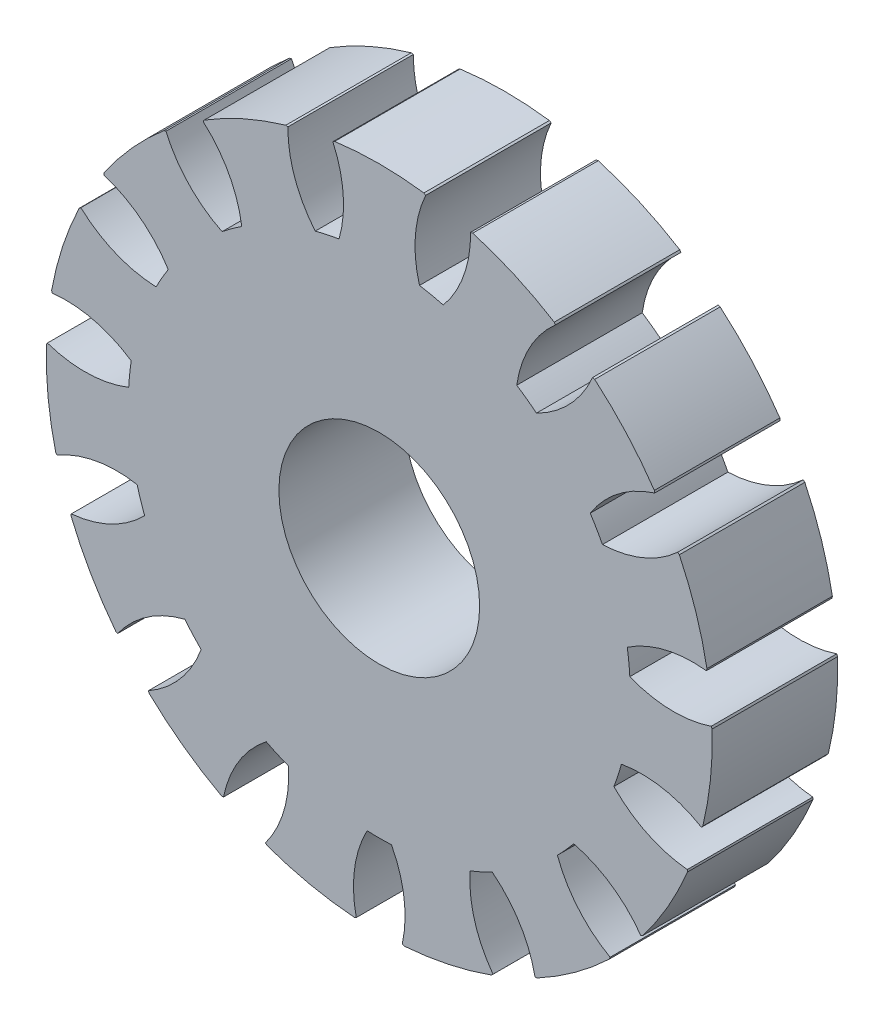
from build123d import *

# Parameters (mm, degrees)
SKETCH1_R           = 10
BOSS_EXTRUDE1_DEPTH = 5
SKETCH4_R           = 2.25
CUT_EXTRUDE2_DEPTH  = 67.5
BOSS_EXTRUDE3_DEPTH = 5
CIRPATTERN2_COUNT   = 15
SKETCH6_OUTSIDE_W   = 36.97
SKETCH6_OUTSIDE_H   = 36.858
SKETCH6_OUTSIDE_R   = 13.270335227
CUT_EXTRUDE3_DEPTH  = 20.926845935
SKETCH7_R           = 4
CUT_EXTRUDE4_DEPTH  = 20.421729945


with BuildPart() as part:
    # Sketch1 → Boss-Extrude1 (new body)
    with BuildSketch(Plane.XY):
        Circle(SKETCH1_R)
    extrude(amount=BOSS_EXTRUDE1_DEPTH)

    # Sketch4 → Cut-Extrude2 (cut, symmetric)
    with BuildSketch(Plane.XY):
        Circle(SKETCH4_R)
    extrude(amount=CUT_EXTRUDE2_DEPTH, both=True, mode=Mode.SUBTRACT)

    # Sketch5 → Boss-Extrude3 (add)
    with BuildSketch(Plane.XY):
        with BuildLine():
            ThreePointArc((1.602050877, 9.870837502), (0, 10), (-1.602050877, 9.870837502))
            ThreePointArc((-1.602050877, 9.870837502), (-1.43729136, 11.509422675), (-1.849699914, 13.103795985))
            ThreePointArc((-1.849699914, 13.103795985), (0, 13.667962875), (1.849699914, 13.103795985))
            ThreePointArc((1.849699914, 13.103795985), (1.43729136, 11.509422675), (1.602050877, 9.870837502))
        make_face()
    boss_extrude3 = extrude(amount=BOSS_EXTRUDE3_DEPTH)

    # CirPattern2: Boss-Extrude3 ×15 about axis
    cirpattern2_axis = Axis((0, 0, 0), (0, 0, 1))
    for i in range(1, CIRPATTERN2_COUNT):
        add(boss_extrude3.rotate(cirpattern2_axis, i * 360 / CIRPATTERN2_COUNT))

    # Sketch6 outside → Cut-Extrude3 (cut, through all)
    with BuildSketch(Plane.XY):
        with Locations((0, 0.113)):
            Rectangle(SKETCH6_OUTSIDE_W, SKETCH6_OUTSIDE_H)
        Circle(SKETCH6_OUTSIDE_R, mode=Mode.SUBTRACT)
    extrude(amount=CUT_EXTRUDE3_DEPTH, mode=Mode.SUBTRACT)

    # Sketch7 → Cut-Extrude4 (cut, through all)
    with BuildSketch(Plane.XY.offset(5)):
        Circle(SKETCH7_R)
    extrude(amount=-CUT_EXTRUDE4_DEPTH, mode=Mode.SUBTRACT)


solid = part.part
